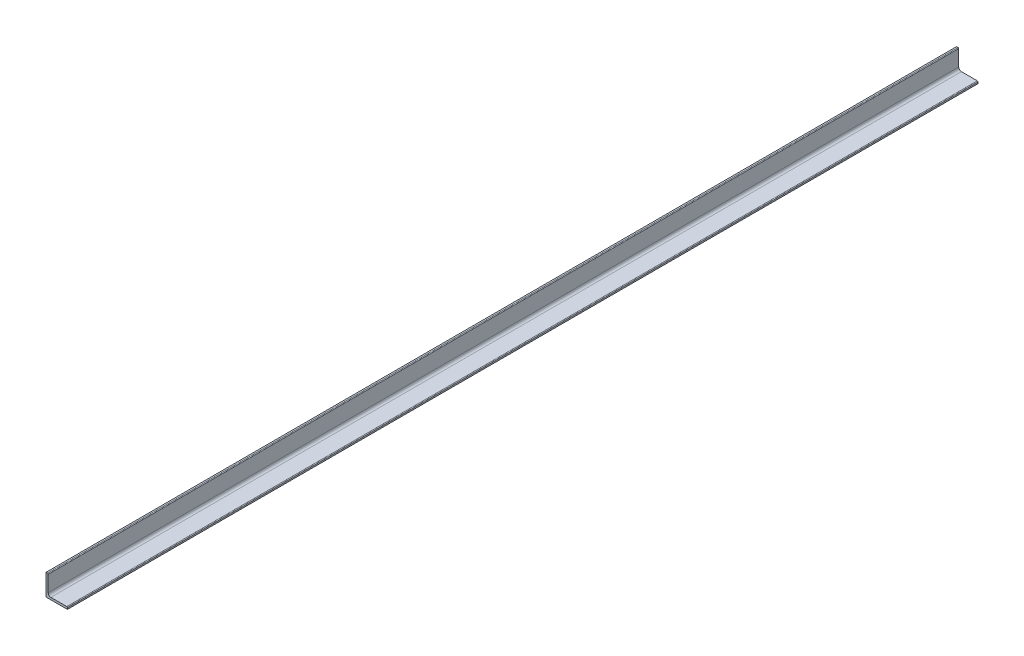
from build123d import *

# Parameters (mm, degrees)
BOSS_EXTRUDE1_DEPTH = 1700


with BuildPart() as part:
    # Sketch1 → Boss-Extrude1 (new body)
    with BuildSketch(Plane.XY):
        with BuildLine():
            Line((0, 0), (0, 40))
            Line((0, 40), (2.666666667, 40))
            ThreePointArc((2.666666667, 40), (3.609475708, 39.609475708), (4, 38.666666667))
            Line((4, 38.666666667), (4, 9))
            ThreePointArc((4, 9), (5.464466094, 5.464466094), (9, 4))
            Line((9, 4), (38.666666667, 4))
            ThreePointArc((38.666666667, 4), (39.609475708, 3.609475708), (40, 2.666666667))
            Line((40, 2.666666667), (40, 0))
            Line((40, 0), (0, 0))
        make_face()
    extrude(amount=BOSS_EXTRUDE1_DEPTH)


solid = part.part
